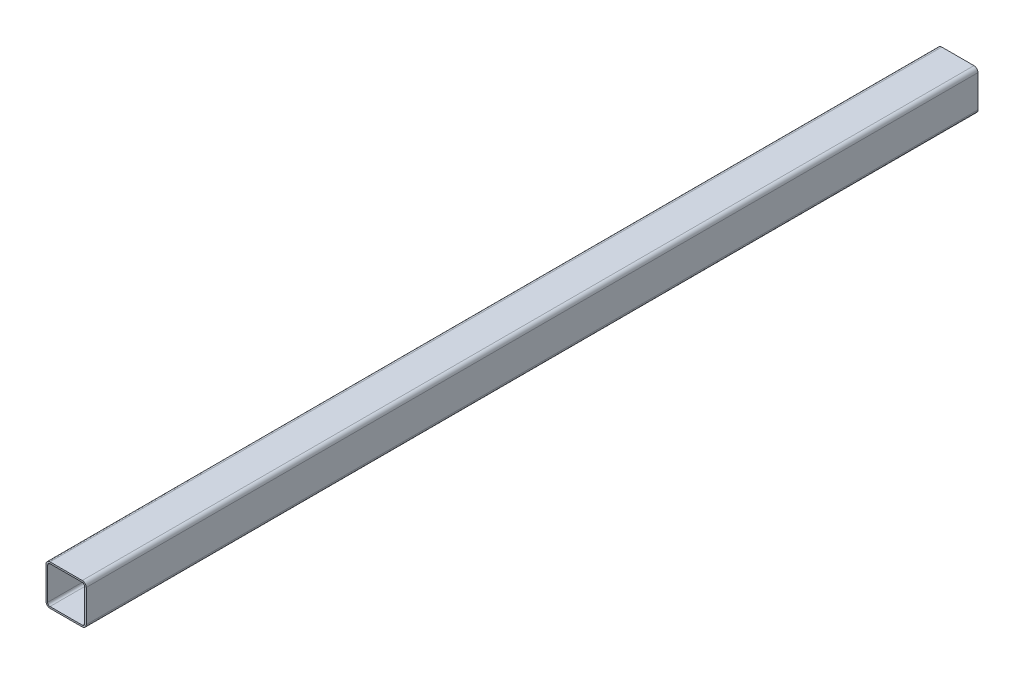
SolidWorks part; units mm, degrees
ref_plane "Front Plane" through (0, 0, 0) normal (0, 0, 1) x (1, 0, 0)
ref_plane "Top Plane" through (0, 0, 0) normal (0, 1, 0) x (1, 0, 0)
ref_plane "Right Plane" through (0, 0, 0) normal (1, 0, 0) x (0, 0, -1)
other "Configuration Table"
sketch "Sketch1" plane through (0, 0, 0) normal (0, 0, 1) x (1, 0, 0)
  line L0 (-92, 80) -> (-92, -80)
  line L1 (-80, 100) -> (80, 100)
  line L2 (-100, 80) -> (-100, -80)
  line L3 (-80, -100) -> (80, -100)
  line L4 (100, 80) -> (100, -80)
  line L5 (-100, 100) -> (100, -100) construction
  line L6 (-100, -100) -> (100, 100) construction
  line L7 (-80, -92) -> (80, -92)
  line L8 (92, 80) -> (92, -80)
  line L9 (-80, 92) -> (80, 92)
  arc A0 (-100, -80) -> (-80, -100) centre (-80, -80) ccw
  arc A1 (80, -100) -> (100, -80) centre (80, -80) ccw
  arc A2 (80, 100) -> (100, 80) centre (80, 80) cw
  arc A3 (-80, 100) -> (-100, 80) centre (-80, 80) ccw
  arc A4 (-92, -80) -> (-80, -92) centre (-80, -80) ccw
  arc A5 (80, -92) -> (92, -80) centre (80, -80) ccw
  arc A6 (80, 92) -> (92, 80) centre (80, 80) cw
  arc A7 (-80, 92) -> (-92, 80) centre (-80, 80) ccw
  point P0 (0, 0)
  dimension "D3" = 20
  dimension "D1" = 200
  dimension "D2" = 200
  dimension "D4" = 8
extrude "Boss-Extrude1" add sketch "Sketch1" along normal blind 4430
